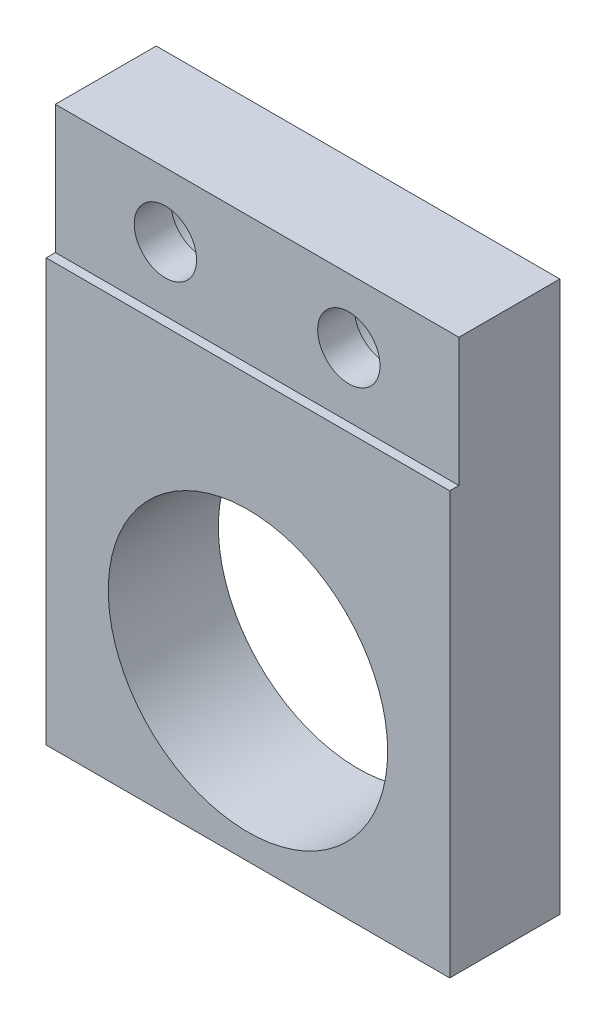
SolidWorks part; units mm, degrees
ref_plane "前视基准面" through (0, 0, 0) normal (0, 0, 1) x (1, 0, 0)
ref_plane "上视基准面" through (0, 0, 0) normal (0, 1, 0) x (1, 0, 0)
ref_plane "右视基准面" through (0, 0, 0) normal (1, 0, 0) x (0, 0, -1)
sketch "草图1" plane through (0, 0, 0) normal (0, 0, 1) x (1, 0, 0)
  line L1 (-12.9358, 14.1193) -> (9.0642, 14.1193)
  line L2 (-12.9358, 14.1193) -> (-12.9358, -15.8807)
  line L3 (-12.9358, -15.8807) -> (9.0642, -15.8807)
  line L4 (9.0642, 14.1193) -> (9.0642, -15.8807)
  circle A0 centre (-1.9358, -6.8807) radius 7.615
  circle A1 centre (-6.9358, 10.6193) radius 1.7
  circle A2 centre (3.0642, 10.6193) radius 1.7
  dimension "D4" = 15.23
  dimension "D7" = 3.4
  dimension "D10" = 3.4
  dimension "D1" = 30
  dimension "D2" = 22
  dimension "D3" = 9
  dimension "D5" = 3.5
  dimension "D6" = 6
  dimension "D8" = 3.5
  dimension "D9" = 6
extrude "凸台-拉伸1" add sketch "草图1" along normal blind 6
sketch "草图3" plane through (-12.9358, 0, 0) normal (-1, 0, 0) x (0, 0, 1)
  line L1 (6, 14.1193) -> (5.5, 14.1193)
  line L2 (6, 14.1193) -> (6, 7.1193)
  line L3 (6, 7.1193) -> (5.5, 7.1193)
  line L4 (5.5, 14.1193) -> (5.5, 7.1193)
  dimension "D1" = 0.5
  dimension "D2" = 7
extrude "切除-拉伸1" cut sketch "草图3" against normal through all
sketch "草图4" plane through (0, 0, 0) normal (0, 0, -1) x (-1, 0, 0)
  circle A0 centre (-3.0642, 10.6193) radius 3
  circle A1 centre (6.9358, 10.6193) radius 3
  dimension "D1" = 6
  dimension "D2" = 6
extrude "切除-拉伸2" cut sketch "草图4" against normal blind 3.5
